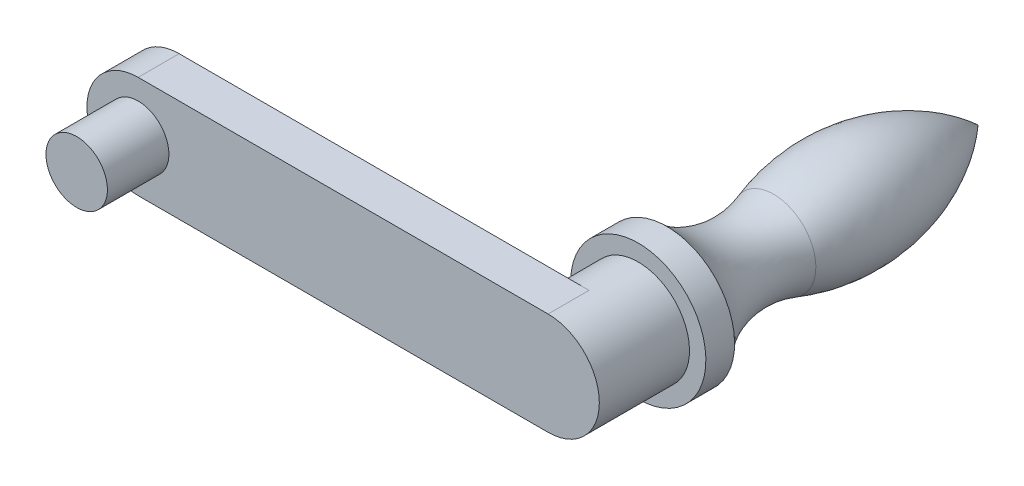
from build123d import *

# Parameters (mm, degrees)
EXTRUDE_1_DEPTH = 10
SKETCH_2_R      = 7.5
EXTRUDE_2_DEPTH = 15


with BuildPart() as part:
    # 草图1 → 凸台-拉伸1 (new body)
    with BuildSketch(Plane.XY):
        with BuildLine():
            Line((0, 0), (100, 0))
            ThreePointArc((100, 0), (112.5, 12.5), (100, 25))
            Line((100, 25), (0, 25))
            ThreePointArc((0, 25), (-12.5, 12.5), (0, 0))
        make_face()
    extrude(amount=EXTRUDE_1_DEPTH)

    # 草图2 → 凸台-拉伸2 (add)
    with BuildSketch(Plane.XY.offset(10)):
        with Locations((0, 12.5)):
            Circle(SKETCH_2_R)
    extrude(amount=EXTRUDE_2_DEPTH)

    # 草图7 → 旋转1 (revolve)
    with BuildSketch(Plane(origin=(100, 0, 0), x_dir=(0, 0, -1), z_dir=(1, 0, 0)), mode=Mode.PRIVATE) as revolve_1_sk:
        with BuildLine():
            Line((0, 12.5), (0, 25))
            Line((0, 25), (12, 25))
            Line((12, 25), (12, 29))
            Line((12, 29), (19, 29))
            ThreePointArc((19, 29), (31.116731463, 22.12336259), (45.032630645, 22.794982573))
            ThreePointArc((45.032630645, 22.794982573), (71.367513527, 24.466816677), (94.885940011, 12.5))
            Line((94.885940011, 12.5), (0, 12.5))
        make_face()
    revolve(revolve_1_sk.sketch.rotate(Axis((100, 12.5, 0), (0, 0, -1)), 180), axis=Axis((100, 12.5, 0), (0, 0, -1)))


solid = part.part
